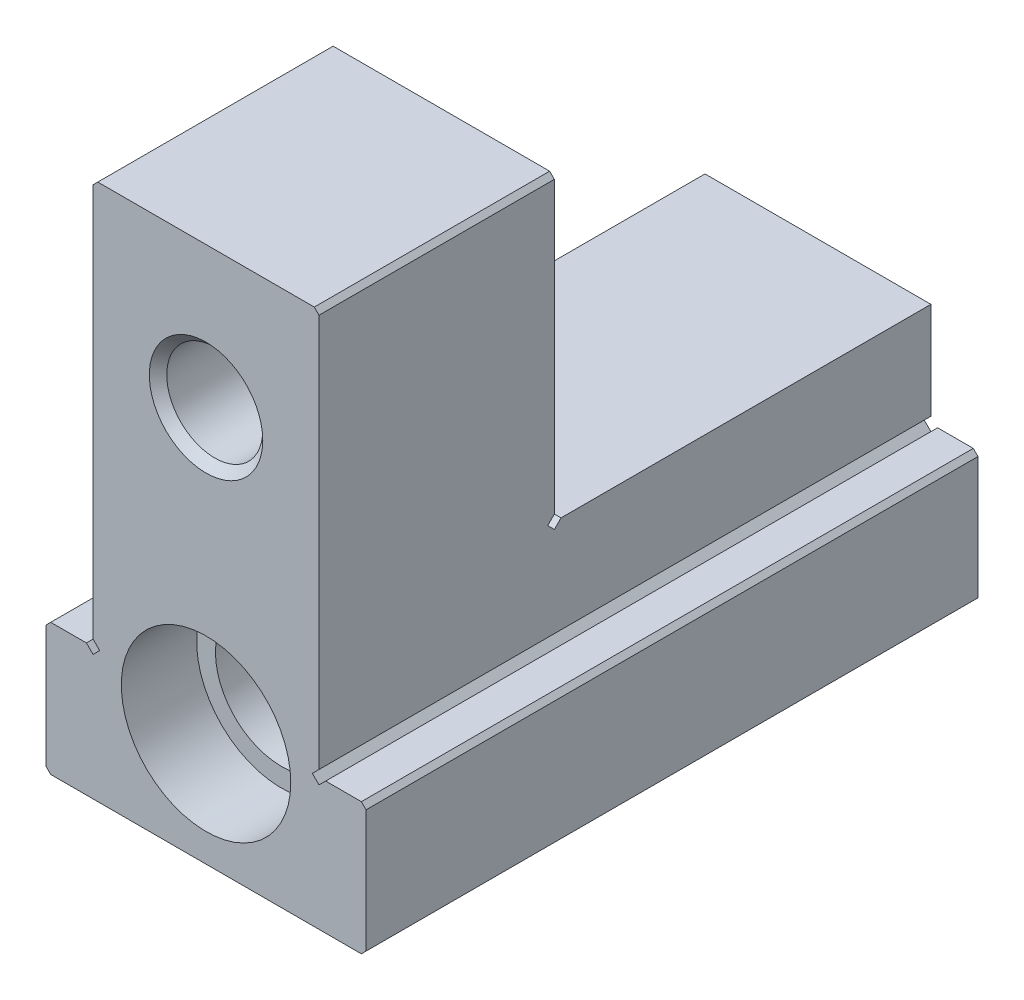
SolidWorks part; units mm, degrees
ref_plane "Front Plane" through (0, 0, 0) normal (0, 0, 1) x (1, 0, 0)
ref_plane "Top Plane" through (0, 0, 0) normal (0, 1, 0) x (1, 0, 0)
ref_plane "Right Plane" through (0, 0, 0) normal (1, 0, 0) x (0, 0, -1)
sketch "Sketch1" plane through (0, 0, 0) normal (0, 0, 1) x (1, 0, 0)
  line L0 (0, 0) -> (0, 57) construction
  line L1 (16.5, 0) -> (-16.5, 0)
  line L2 (-17, 0.5) -> (-17, 13.5)
  line L3 (-16.5, 14) -> (-12.7071, 14)
  line L4 (-12, 14.7071) -> (-12, 56.5)
  line L5 (-11.5, 57) -> (11.5, 57)
  line L6 (-12, 56.5) -> (-11.5, 57)
  line L7 (-17, 13.5) -> (-16.5, 14)
  line L8 (-16.5, 0) -> (-17, 0.5)
  line L9 (-12, 14) -> (-16.1123, 18.1123) construction
  line L10 (-12.7071, 14) -> (-12, 13.2929)
  line L11 (-12, 14.7071) -> (-11.2929, 14)
  line L12 (-12, 13.2929) -> (-11.2929, 14)
  line L13 (12, 14) -> (16.1123, 18.1123) construction
  line L14 (12, 13.2929) -> (11.2929, 14)
  line L15 (12, 14.7071) -> (11.2929, 14)
  line L16 (12.7071, 14) -> (12, 13.2929)
  line L17 (16.5, 0) -> (17, 0.5)
  line L18 (17, 13.5) -> (16.5, 14)
  line L19 (12, 56.5) -> (11.5, 57)
  line L20 (12, 14.7071) -> (12, 56.5)
  line L21 (16.5, 14) -> (12.7071, 14)
  line L22 (17, 0.5) -> (17, 13.5)
  point P4 (-17, 0)
  point P5 (-17, 14)
  point P7 (-12, 57)
  point P30 (12, 57)
  point P31 (17, 14)
  point P32 (17, 0)
  dimension "D1" = 57
  dimension "D2" = 17
  dimension "D3" = 12
  dimension "D4" = 14
  dimension "D5" = 45
  dimension "D6" = 1
  dimension "D10" = 0.5
  dimension "D11" = 1
extrude "Boss-Extrude1" add sketch "Sketch1" along normal blind 65
sketch "Sketch2" plane through (12, 0, 0) normal (1, 0, 0) x (0, 0, -1)
  line L0 (-65, 14.7071) -> (-65, 56.5) construction
  line L1 (-40, 79.7152) -> (7.536, 79.7152)
  line L2 (-40, 79.7152) -> (-40, 25.7071)
  line L3 (-39.2929, 25) -> (7.536, 25)
  line L4 (7.536, 79.7152) -> (7.536, 25)
  line L5 (-40, 25) -> (-30.929, 34.071) construction
  line L6 (-40, 25.7071) -> (-40.7071, 25)
  line L7 (-40.7071, 25) -> (-40, 24.2929)
  line L8 (-40, 24.2929) -> (-39.2929, 25)
  dimension "D1" = 25
  dimension "D2" = 25
  dimension "D3" = 45
  dimension "D4" = 1
  dimension "D5" = 0.5
  dimension "D6" = 1
extrude "Cut-Extrude1" cut sketch "Sketch2" against normal through all both and the other way through all
sketch "Sketch3" plane through (0, 0, 65) normal (0, 0, 1) x (1, 0, 0)
  line L0 (-16.5, 0) -> (16.5, 0) construction
  line L1 (0, 0) -> (0, 12) construction
  circle A0 centre (0, 12) radius 9
  dimension "D1" = 18
  dimension "D2" = 12
extrude "Cut-Extrude2" cut sketch "Sketch3" against normal blind 8
sketch "Sketch4" plane through (0, 0, 0) normal (0, 0, -1) x (-1, 0, 0)
  line L0 (16.5, 0) -> (-16.5, 0) construction
  circle A0 centre (0, 12) radius 9
  dimension "D1" = 12
  dimension "D2" = 18
extrude "Cut-Extrude3" cut sketch "Sketch4" against normal blind 8
hole_wizard "M16 Tapped Hole1" positions "3DSketch1" profile "Sketch5" tap size "M16" standard "GB" end condition through all
sketch3d "3DSketch1"
  line L0 (0, 12, 8) -> (0, 12, 0) construction
  point P0 (0, 12, 8)
sketch "Sketch5" plane through (0, 12, 8) normal (1, 0, 0) x (0, 1, 0)
  line L0 (0, 0) -> (0, 57)
  line L1 (0, 57) -> (7, 57)
  line L2 (7, 57) -> (7, 1.025)
  line L3 (7, 1.025) -> (8.025, 0)
  line L5 (8.025, 0) -> (0, 0)
  line L6 (-7, 1.025) -> (-8.025, 0) construction
  line L11 (0, -6.35) -> (0, 107.95) construction
  dimension "通孔螺纹孔钻头直径" = 14
  dimension "通孔螺纹孔钻头深度" = 57
  dimension "近端锥形沉头孔直径" = 16.05
  dimension "近端锥形沉头孔角度" = 90
cosmetic thread "Hole thread 1" parameters "D2"=16
hole_wizard "M12 Tapped Hole1" positions "3DSketch2" profile "Sketch6" tap size "M12" standard "GB" end condition through all
sketch3d "3DSketch2"
  line L0 (11.5, 57, 65) -> (-11.5, 57, 65) construction
  point P0 (0, 42, 65)
  dimension "D1" = 15
  dimension "D2" = 12
sketch "Sketch6" plane through (0, 42, 65) normal (1, 0, 0) x (0, -1, 0)
  line L0 (0, 0) -> (0, 65)
  line L1 (0, 65) -> (5.1, 65)
  line L2 (5.1, 65) -> (5.1, 0.925)
  line L3 (5.1, 0.925) -> (6.025, 0)
  line L5 (6.025, 0) -> (0, 0)
  line L6 (-5.1, 0.925) -> (-6.025, 0) construction
  line L11 (0, -6.35) -> (0, 107.95) construction
  dimension "通孔螺纹孔钻头直径" = 10.2
  dimension "通孔螺纹孔钻头深度" = 65
  dimension "近端锥形沉头孔直径" = 12.05
  dimension "近端锥形沉头孔角度" = 90
cosmetic thread "Hole thread 2" parameters "D2"=12
